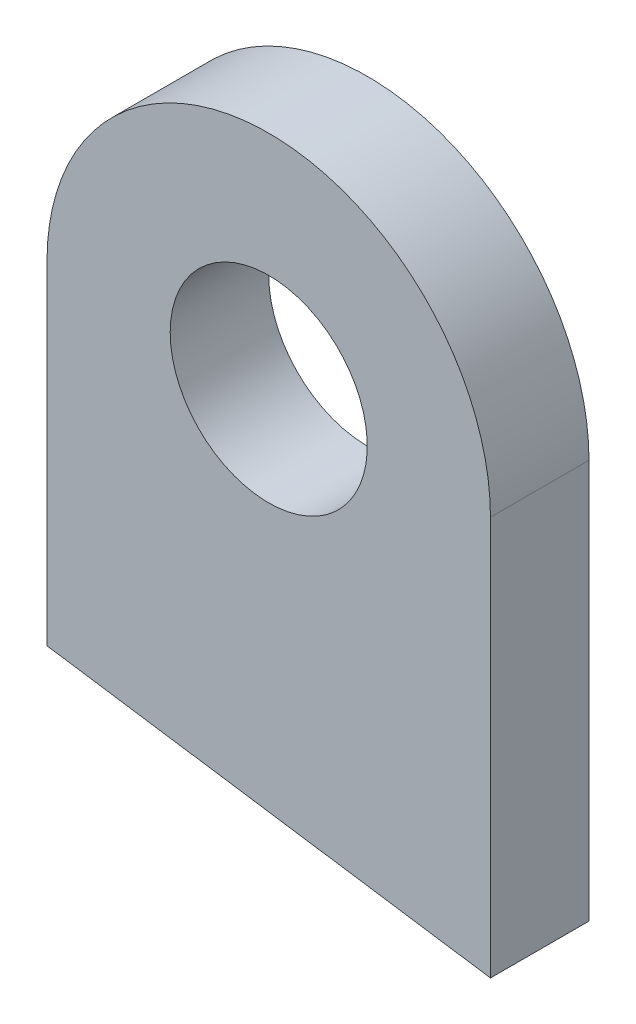
from build123d import *

# Parameters (mm, degrees)
EXTRUDE_1_DEPTH     = 20
SKETCH_2_R          = 20
CUT_EXTRUDE_1_DEPTH = 157.12815249


with BuildPart() as part:
    # 草图1 → 凸台-拉伸1 (new body)
    with BuildSketch(Plane.XY):
        with BuildLine():
            Line((0, 0), (0, 81))
            ThreePointArc((0, 81), (-45, 126), (-90, 81))
            Line((-90, 81), (-90, 13.383545734))
            Line((-90, 13.383545734), (0, 0))
        make_face()
    extrude(amount=EXTRUDE_1_DEPTH)

    # 草图2 → 切除-拉伸1 (cut, through all)
    with BuildSketch(Plane(origin=(0, 0, 0), x_dir=(-1, 0, 0), z_dir=(0, 0, -1))):
        with Locations((45, 81)):
            Circle(SKETCH_2_R)
    extrude(amount=-CUT_EXTRUDE_1_DEPTH, mode=Mode.SUBTRACT)


solid = part.part
